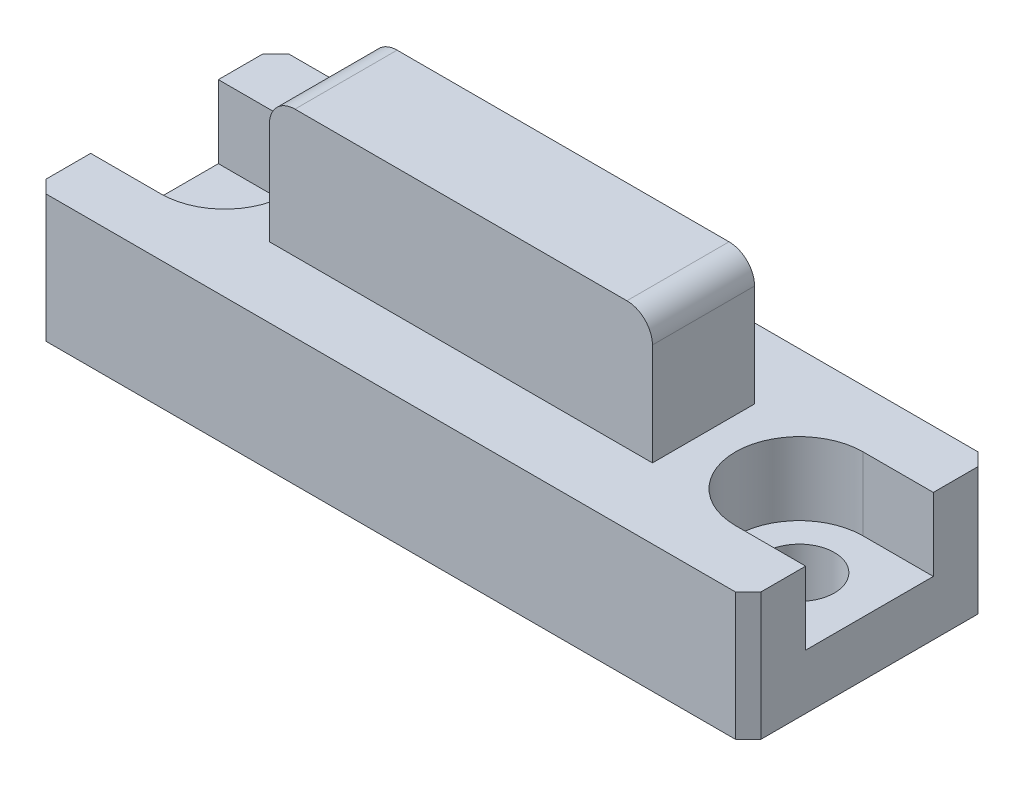
SolidWorks part; units mm, degrees
ref_plane "Front Plane" through (0, 0, 0) normal (0, 0, 1) x (1, 0, 0)
ref_plane "Top Plane" through (0, 0, 0) normal (0, 1, 0) x (1, 0, 0)
ref_plane "Right Plane" through (0, 0, 0) normal (1, 0, 0) x (0, 0, -1)
sketch "Sketch1" plane through (0, 0, 0) normal (0, 0, 1) x (1, 0, 0)
  line L0 (0, 0) -> (0, 29.9664) construction
  line L1 (28, 0) -> (-28, 0)
  line L2 (-28, 0) -> (-28, 10)
  line L3 (-28, 10) -> (-15, 10)
  line L4 (-15, 10) -> (-15, 20)
  line L5 (-15, 20) -> (15, 20)
  line L6 (15, 10) -> (15, 20)
  line L7 (28, 10) -> (15, 10)
  line L8 (28, 0) -> (28, 10)
  point P9 (0, 20)
  dimension "D1" = 56
  dimension "D2" = 30
  dimension "D3" = 10
  dimension "D4" = 20
extrude "Boss-Extrude1" add sketch "Sketch1" along normal mid plane 19
hole_wizard "Hole size per socket head cap screw type 1" positions "Sketch3" profile "Sketch2" counterbore size "M5" standard "GB" end condition through all
sketch "Sketch3" plane through (0, 10, 0) normal (0, 1, 0) x (-1, 0, 0)
  line L0 (22.5, 0) -> (-22.5, 0) construction
  point P0 (22.5, 0)
  point P1 (-22.5, 0)
  dimension "D1" = 45
sketch "Sketch2" plane through (-22.5, 10, 0) normal (1, 0, 0) x (0, 0, 1)
  line L0 (0, 0) -> (0, 10)
  line L1 (0, 10) -> (2.75, 10)
  line L3 (2.75, 10) -> (2.75, 5.7)
  line L4 (2.75, 5.7) -> (5, 5.7)
  line L5 (5, 5.7) -> (5, 0)
  line L7 (5, 0) -> (0, 0)
  line L11 (0, -6.35) -> (0, 107.95) construction
  dimension "通孔孔直径" = 5.5
  dimension "通孔孔深度" = 10
  dimension "柱形沉头孔直径" = 10
  dimension "柱形沉头孔深度" = 5.7
sketch "Sketch4" plane through (0, 10, 0) normal (0, 1, 0) x (1, 0, 0)
  line L0 (-28, -9.5) -> (-28, 9.5) construction
  line L1 (-28, -5) -> (-22.5, -5)
  line L2 (-28, -5) -> (-28, 5)
  line L3 (-28, 5) -> (-22.5, 5)
  line L4 (-22.5, -5) -> (-22.5, 5)
  line L5 (-22.5, 0) -> (-22.5, -5) construction
  line L6 (22.5, 0) -> (22.5, -5) construction
  line L7 (28, -9.5) -> (28, 9.5) construction
  line L8 (22.5, -5) -> (28, -5)
  line L9 (22.5, -5) -> (22.5, 5)
  line L10 (22.5, 5) -> (28, 5)
  line L11 (28, -5) -> (28, 5)
  circle A0 centre (-22.5, 0) radius 5 construction
  circle A1 centre (-22.5, 0) radius 5 construction
  circle A3 centre (22.5, 0) radius 5 construction
  circle A4 centre (22.5, 0) radius 5 construction
extrude "Cut-Extrude1" cut sketch "Sketch4" against normal up to surface (5.7 mm away) up to face at (-22.5, 4.3, 2.75)
sketch "Sketch5" plane through (0, 20, 0) normal (0, 1, 0) x (1, 0, 0)
  line L1 (15, 9.5) -> (-15, 9.5) construction
  line L2 (-15, 15) -> (15, 15)
  line L3 (-15, 15) -> (-15, 4)
  line L4 (-15, 4) -> (15, 4)
  line L5 (15, 15) -> (15, 4)
  line L6 (-15, 15) -> (15, 4) construction
  line L7 (-15, 4) -> (15, 15) construction
  line L8 (15, -9.5) -> (15, 9.5) construction
  line L9 (15, -9.5) -> (-15, -9.5) construction
  line L10 (-15, -15) -> (15, -15)
  line L11 (-15, -15) -> (-15, -4)
  line L12 (-15, -4) -> (15, -4)
  line L13 (15, -15) -> (15, -4)
  line L14 (-15, -15) -> (15, -4) construction
  line L15 (-15, -4) -> (15, -15) construction
  line L16 (15, -9.5) -> (15, 9.5) construction
  point P0 (0, 9.5)
  point P10 (0, -9.5)
  dimension "D1" = 8
  dimension "D2" = 4
extrude "Cut-Extrude2" cut sketch "Sketch5" against normal up to surface (10 mm away) up to face at (-22.75, 10, 0)
chamfer "Chamfer1" distance 1 angle 45 4 edges at (28, 5, 9.5) (28, 5, -9.5) (-28, 5, -9.5) (-28, 5, 9.5)
fillet "Fillet1" radius 2 2 edges at (15, 20, 0) (-15, 20, 0)
